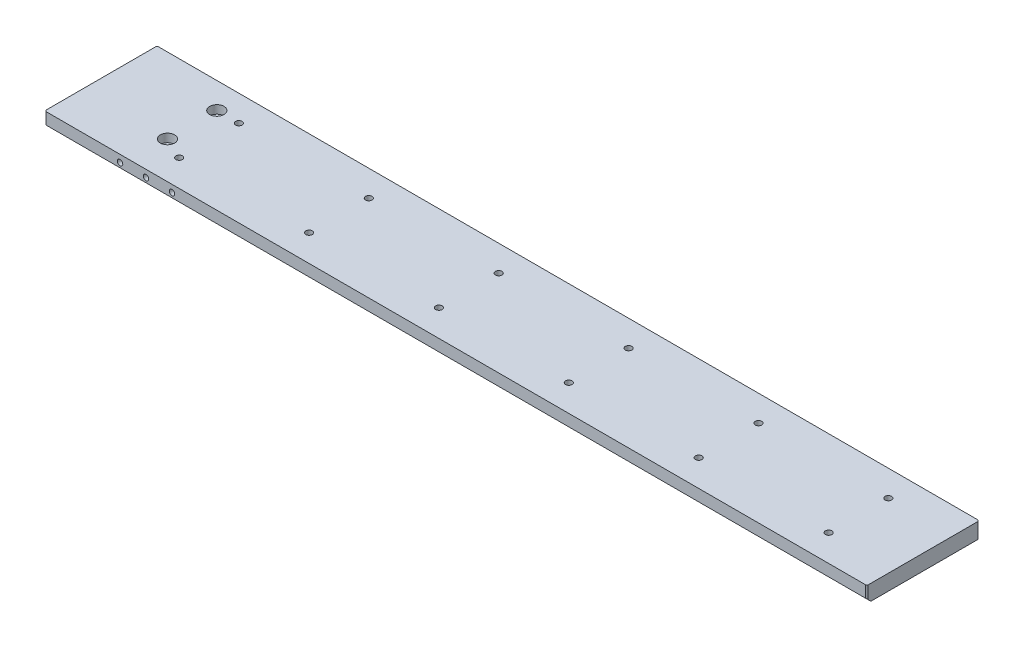
from build123d import *

# Parameters (mm, degrees)
SKETCH_1_W                     = 800
SKETCH_1_H                     = 80
EXTRUDE_1_DEPTH                = 12
SKETCH_13_W                    = 10
SKETCH_13_H                    = 40
EXTRUDE_2_DEPTH                = 800
CUT_EXTRUDE_1_DEPTH            = 409.881400898
CUT_EXTRUDE_1_DEPTH_BACK       = 409.881400898
SKETCH_15_W                    = 47
SKETCH_15_H                    = 70
CUT_EXTRUDE_2_DEPTH            = 403.968981437
CUT_EXTRUDE_3_DEPTH            = 665.795457265
CUT_EXTRUDE_3_DEPTH_BACK       = 665.795457265
CUT_EXTRUDE_4_DEPTH            = 665.795457265
CUT_EXTRUDE_4_DEPTH_BACK       = 665.795457265
PATTERN_LINEAR_1_COUNT         = 7
PATTERN_LINEAR_1_PITCH         = 82
HOLE_WIZARD_M6_1_2_D           = 6.6
HOLE_WIZARD_M6_1_2_CBORE_D     = 11
HOLE_WIZARD_M6_1_2_CBORE_DEPTH = 6.4
HOLE_WIZARD_5_0_5_1_D          = 5
HOLE_WIZARD_5_0_5_1_DEPTH      = 10
HOLE_WIZARD_5_0_5_1_TIP        = 1.443375673
CUT_EXTRUDE_5_DEPTH            = 10
SKETCH_26_W                    = 663
SKETCH_26_H                    = 18.5
EXTRUDE_3_DEPTH                = 12
CHAMFER_1_SIZE                 = 3
HOLE_WIZARD_M6_2_AT_2_COUNT    = 2
HOLE_WIZARD_M6_2_AT_2_PITCH    = 46
PATTERN_LINEAR_2_COUNT         = 6
PATTERN_LINEAR_2_PITCH         = 100
HOLE_WIZARD_M5_1_D             = 4.2
HOLE_WIZARD_M5_1_DEPTH         = 12.4
HOLE_WIZARD_M5_1_TIP           = 1.2618073
CUT_EXTRUDE_6_DEPTH            = 410.421842126
CUT_EXTRUDE_6_DEPTH_BACK       = 410.421842126
CHAMFER_2_SIZE                 = 1


with BuildPart() as part:
    # 草图1 → 凸台-拉伸1 (new body)
    with BuildSketch(Plane(origin=(0, 0, 0), x_dir=(1, 0, 0), z_dir=(0, 1, 0))):
        Rectangle(SKETCH_1_W, SKETCH_1_H)
    extrude(amount=EXTRUDE_1_DEPTH)

    # 草图13 → 凸台-拉伸2 (add)
    with BuildSketch(Plane(origin=(400, 0, 0), x_dir=(0, 0, -1), z_dir=(1, 0, 0))):
        with Locations((35, -8)):
            Rectangle(SKETCH_13_W, SKETCH_13_H)
    extrude(amount=-EXTRUDE_2_DEPTH)

    # 草图14 → 切除-拉伸1 (cut, two sides: drawn at the far end of the back side and taken through both)
    with BuildSketch(Plane.XY.offset(40).offset(-CUT_EXTRUDE_1_DEPTH_BACK)):
        Polygon((310, 1445.673153531), (310, 12), (310, -39.100998243), (310, -1472.774151774), (3177.346307063, -1472.774151774), (3177.346307063, 1445.673153531), align=None)
    extrude(amount=CUT_EXTRUDE_1_DEPTH + CUT_EXTRUDE_1_DEPTH_BACK, mode=Mode.SUBTRACT)

    # 草图15 → 切除-拉伸2 (cut, through all)
    with BuildSketch(Plane.XZ):
        with Locations((286.5, 5)):
            Rectangle(SKETCH_15_W, SKETCH_15_H)
    extrude(amount=-CUT_EXTRUDE_2_DEPTH, mode=Mode.SUBTRACT)

    # 草图16 → 切除-拉伸3 (cut, two sides: drawn at the far end of the back side and taken through both)
    with BuildSketch(Plane(origin=(263, 0, 0), x_dir=(0, 0, -1), z_dir=(1, 0, 0)).offset(-CUT_EXTRUDE_3_DEPTH_BACK)):
        Polygon((-37.99997, 201.49334526), (-37.99997, 14.161837787), (-37.99997, -5.873299283), (-37.99997, -193.204806756), (-412.662984945, -193.204806756), (-412.662984945, 201.49334526), align=None)
    extrude(amount=CUT_EXTRUDE_3_DEPTH + CUT_EXTRUDE_3_DEPTH_BACK, mode=Mode.SUBTRACT)

    # 草图17 → 切除-拉伸4 (cut, two sides: drawn at the far end of the back side and taken through both)
    with BuildSketch(Plane(origin=(263, 0, 0), x_dir=(0, 0, -1), z_dir=(1, 0, 0)).offset(-CUT_EXTRUDE_4_DEPTH_BACK)):
        Polygon((30, 179.784611671), (30, 12), (30, -28), (30, -195.784611671), (365.569223341, -195.784611671), (365.569223341, 179.784611671), align=None)
    extrude(amount=CUT_EXTRUDE_4_DEPTH + CUT_EXTRUDE_4_DEPTH_BACK, mode=Mode.SUBTRACT)

    # 草图18 → Hole Wizard M6 _1 (revolve, cut)
    with BuildSketch(Plane(origin=(213, 6, -30), x_dir=(0, 1, 0), z_dir=(1, 0, 0))):
        Polygon((0, 0), (0, 15.502151548), (2.5, 14), (2.5, 0), align=None)
    hole_wizard_m6_1 = revolve(axis=Axis((213, 6, -36.35), (0, 0, 1)), mode=Mode.SUBTRACT)

    # 阵列(线性)1: Hole Wizard M6 _1 ×7
    with Locations(*[(-i * PATTERN_LINEAR_1_PITCH, 0, 0) for i in range(1, PATTERN_LINEAR_1_COUNT)]):
        add(hole_wizard_m6_1, mode=Mode.SUBTRACT)

    # Hole Wizard M6 _1 2 (through all)
    with Locations(Plane(origin=(0, 12, 0), x_dir=(1, 0, 0), z_dir=(0, 1, 0))):
        with Locations((-304, 10), (-304, -28)):
            CounterBoreHole(HOLE_WIZARD_M6_1_2_D / 2, HOLE_WIZARD_M6_1_2_CBORE_D / 2, HOLE_WIZARD_M6_1_2_CBORE_DEPTH)

    # Ø5.0 (5) 直径孔1
    with Locations(Plane(origin=(0, 0, -30), x_dir=(-1, 0, 0), z_dir=(0, 0, -1))):
        with Locations((360, 6)):
            Hole(HOLE_WIZARD_5_0_5_1_D / 2, depth=HOLE_WIZARD_5_0_5_1_DEPTH)
            with Locations((0, 0, -(HOLE_WIZARD_5_0_5_1_DEPTH + HOLE_WIZARD_5_0_5_1_TIP / 2))):  # 120° drill point
                Cone(0, HOLE_WIZARD_5_0_5_1_D / 2, HOLE_WIZARD_5_0_5_1_TIP, mode=Mode.SUBTRACT)

    # 草图24 → 切除-拉伸5 (cut)
    with BuildSketch(Plane(origin=(0, 0, -30), x_dir=(-1, 0, 0), z_dir=(0, 0, -1))):
        with BuildLine():
            Line((-227, 3.5), (-233, 3.5))
            ThreePointArc((-233, 3.5), (-235.5, 6), (-233, 8.5))
            Line((-233, 8.5), (-227, 8.5))
            ThreePointArc((-227, 8.5), (-224.5, 6), (-227, 3.5))
        make_face()
    extrude(amount=-CUT_EXTRUDE_5_DEPTH, mode=Mode.SUBTRACT)

    # 草图26 → 凸台-拉伸3 (add)
    with BuildSketch(Plane.XZ):
        with Locations((-68.5, 47.24997)):
            Rectangle(SKETCH_26_W, SKETCH_26_H)
    extrude(amount=-EXTRUDE_3_DEPTH)

    # 倒角1
    chamfer_1_edges = [part.edges().sort_by_distance(p)[0] for p in [
        (-68.5, 0, 56.49997),
    ]]
    chamfer(chamfer_1_edges, length=CHAMFER_1_SIZE)

    # 草图27 → M6 螺纹孔2 (revolve, cut)
    with BuildSketch(Plane(origin=(213, 12, -10), x_dir=(0, 0, 1), z_dir=(1, 0, 0))):
        Polygon((0, 0), (0, 16.502151548), (2.5, 15), (2.5, 0), align=None)
    hole_wizard_m6_2 = revolve(axis=Axis((213, 18.35, -10), (0, -1, 0)), mode=Mode.SUBTRACT)

    # M6 螺纹孔2 at 2: M6 螺纹孔2 ×2
    with Locations(*[(0, 0, i * HOLE_WIZARD_M6_2_AT_2_PITCH) for i in range(1, HOLE_WIZARD_M6_2_AT_2_COUNT)]):
        add(hole_wizard_m6_2, mode=Mode.SUBTRACT)

    # 阵列(线性)2: M6 螺纹孔2 ×6
    with Locations(*[(-i * PATTERN_LINEAR_2_PITCH, 0, 0) for i in range(1, PATTERN_LINEAR_2_COUNT)]):
        add(hole_wizard_m6_2, mode=Mode.SUBTRACT)

    # 阵列(线性)2 copy 1 sketch → 阵列(线性)2 copy 1 (revolve, cut)
    with BuildSketch(Plane(origin=(113, 12, 36), x_dir=(0, 0, 1), z_dir=(1, 0, 0))):
        Polygon((0, 0), (0, 16.502151548), (2.5, 15), (2.5, 0), align=None)
    revolve(axis=Axis((113, 18.35, 36), (0, -1, 0)), mode=Mode.SUBTRACT)

    # 阵列(线性)2 copy 2 sketch → 阵列(线性)2 copy 2 (revolve, cut)
    with BuildSketch(Plane(origin=(13, 12, 36), x_dir=(0, 0, 1), z_dir=(1, 0, 0))):
        Polygon((0, 0), (0, 16.502151548), (2.5, 15), (2.5, 0), align=None)
    revolve(axis=Axis((13, 18.35, 36), (0, -1, 0)), mode=Mode.SUBTRACT)

    # 阵列(线性)2 copy 3 sketch → 阵列(线性)2 copy 3 (revolve, cut)
    with BuildSketch(Plane(origin=(-87, 12, 36), x_dir=(0, 0, 1), z_dir=(1, 0, 0))):
        Polygon((0, 0), (0, 16.502151548), (2.5, 15), (2.5, 0), align=None)
    revolve(axis=Axis((-87, 18.35, 36), (0, -1, 0)), mode=Mode.SUBTRACT)

    # 阵列(线性)2 copy 4 sketch → 阵列(线性)2 copy 4 (revolve, cut)
    with BuildSketch(Plane(origin=(-187, 12, 36), x_dir=(0, 0, 1), z_dir=(1, 0, 0))):
        Polygon((0, 0), (0, 16.502151548), (2.5, 15), (2.5, 0), align=None)
    revolve(axis=Axis((-187, 18.35, 36), (0, -1, 0)), mode=Mode.SUBTRACT)

    # 阵列(线性)2 copy 5 sketch → 阵列(线性)2 copy 5 (revolve, cut)
    with BuildSketch(Plane(origin=(-287, 12, 36), x_dir=(0, 0, 1), z_dir=(1, 0, 0))):
        Polygon((0, 0), (0, 16.502151548), (2.5, 15), (2.5, 0), align=None)
    revolve(axis=Axis((-287, 18.35, 36), (0, -1, 0)), mode=Mode.SUBTRACT)

    # M5 螺纹孔1
    with Locations(Plane.XY.offset(56.49997)):
        with Locations((-312.000000001, 6.5), (-292.000000001, 6.5), (-272.000000001, 6.5)):
            Hole(HOLE_WIZARD_M5_1_D / 2, depth=HOLE_WIZARD_M5_1_DEPTH)
            with Locations((0, 0, -(HOLE_WIZARD_M5_1_DEPTH + HOLE_WIZARD_M5_1_TIP / 2))):  # 118° drill point
                Cone(0, HOLE_WIZARD_M5_1_D / 2, HOLE_WIZARD_M5_1_TIP, mode=Mode.SUBTRACT)

    # 草图31 → 切除-拉伸6 (cut, two sides: drawn at the far end of the back side and taken through both)
    with BuildSketch(Plane.XY.offset(56.49997).offset(-CUT_EXTRUDE_6_DEPTH_BACK)):
        Polygon((-370, 1306.901366583), (-370, 26.75), (-370, -39.304225055), (-370, -1319.455591638), (-2930.302733167, -1319.455591638), (-2930.302733167, 1306.901366583), align=None)
    extrude(amount=CUT_EXTRUDE_6_DEPTH + CUT_EXTRUDE_6_DEPTH_BACK, mode=Mode.SUBTRACT)

    # 倒角2
    chamfer_2_edges = [part.edges().sort_by_distance(p)[0] for p in [
        (263, 7.5, 56.49997),
        (-370, 6, -30),
        (-370, 7.5, 56.49997),
        (263, 6, -30),
    ]]
    chamfer(chamfer_2_edges, length=CHAMFER_2_SIZE)


solid = part.part
